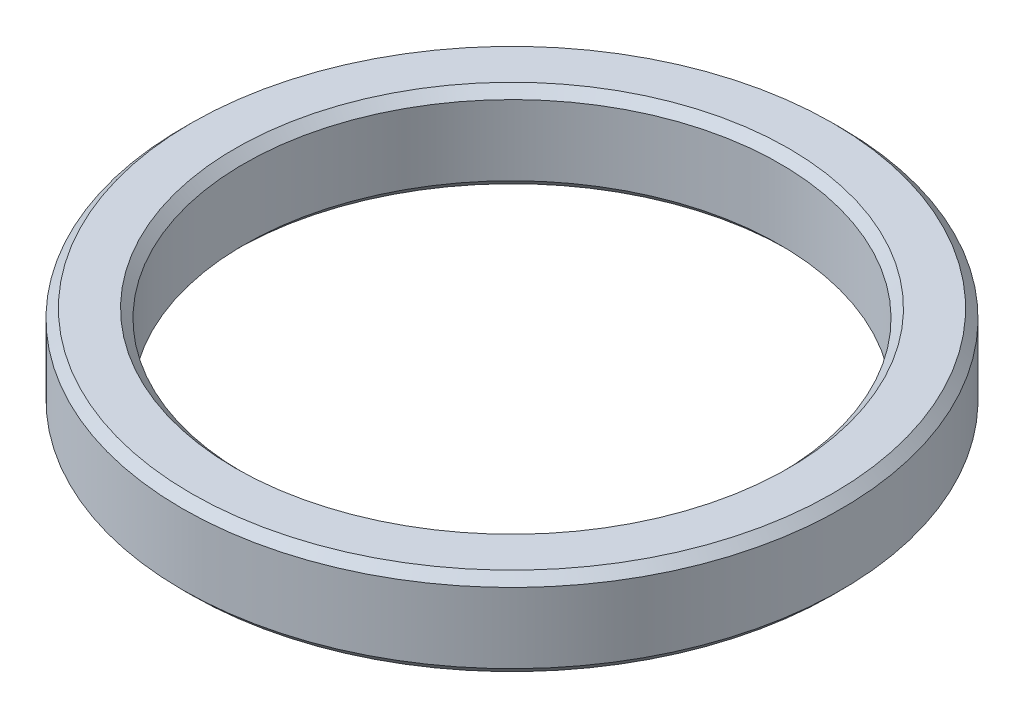
SolidWorks part; units mm, degrees
material "20 steel"
ref_plane "Front Plane" through (0, 0, 0) normal (0, 0, 1) x (1, 0, 0)
ref_plane "Top Plane" through (0, 0, 0) normal (0, 1, 0) x (1, 0, 0)
ref_plane "Right Plane" through (0, 0, 0) normal (1, 0, 0) x (0, 0, -1)
other "Configuration Table"
sketch "Sketch1" plane through (0, 0, 0) normal (0, 1, 0) x (1, 0, 0)
  circle A0 centre (0, 0) radius 37.5
  circle A1 centre (0, 0) radius 30.5
  dimension "D1" = 75
  dimension "D2" = 61
extrude "Boss-Extrude1" add sketch "Sketch1" along normal blind 10
chamfer "Chamfer1" distance 1 angle 45 4 edges at (0, 10, 37.5) (0, 0, 37.5) (0, 10, 30.5) (0, 0, 30.5)
